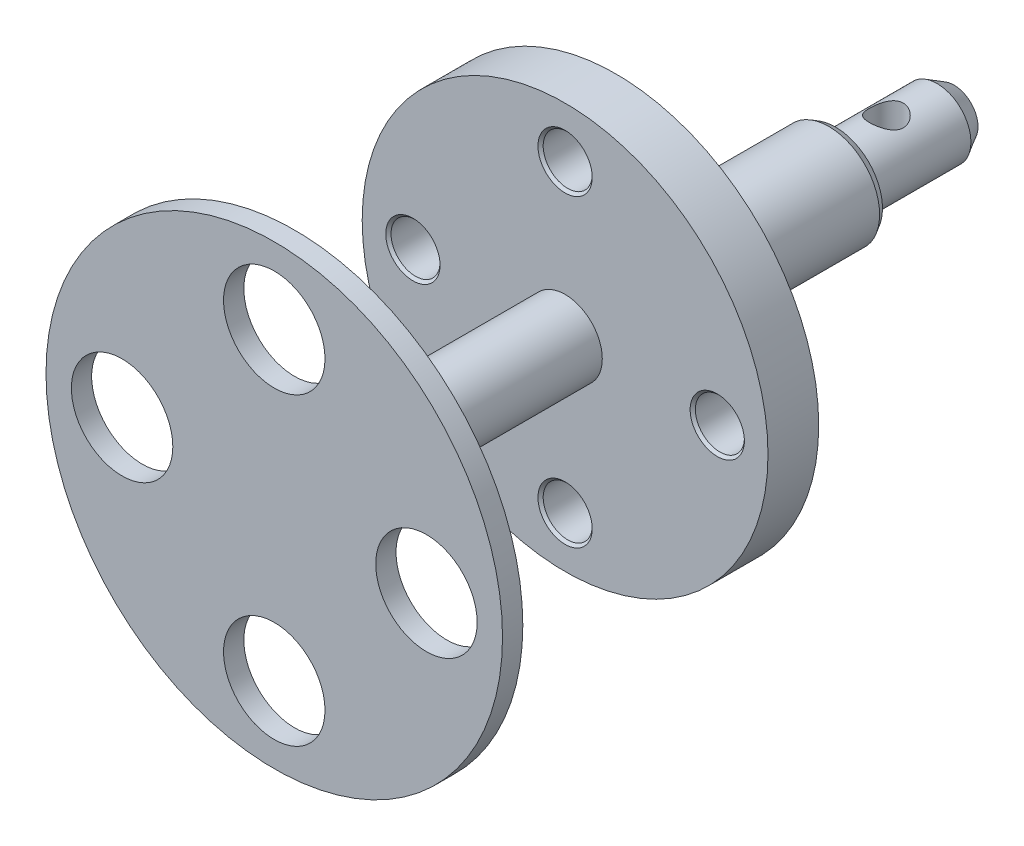
SolidWorks part; units mm, degrees
ref_plane "Front Plane" through (0, 0, 0) normal (0, 0, 1) x (1, 0, 0)
ref_plane "Top Plane" through (0, 0, 0) normal (0, 1, 0) x (1, 0, 0)
ref_plane "Right Plane" through (0, 0, 0) normal (1, 0, 0) x (0, 0, -1)
other "Configuration Table"
sketch "Sketch1" plane through (0, 0, 0) normal (0, 0, 1) x (1, 0, 0)
  circle A0 centre (0, 0) radius 52.5
  circle A1 centre (0, 0) radius 45 construction
  circle A2 centre (0, 45) radius 3.5
  circle A3 centre (38.9711, 22.5) radius 3.5
  circle A4 centre (38.9711, -22.5) radius 3.5
  circle A5 centre (0, -45) radius 3.5
  circle A6 centre (-38.9711, -22.5) radius 3.5
  circle A7 centre (-38.9711, 22.5) radius 3.5
  point P19 (0, 0)
  dimension "D1" = 105
  dimension "D2" = 90
  dimension "D3" = 7
  dimension "D4" = 6
extrude "Boss-Extrude1" add sketch "Sketch1" along normal blind 14
sketch "Sketch2" plane through (0, 0, 14) normal (0, 0, 1) x (1, 0, 0)
  circle A1 centre (0, 0) radius 10
  dimension "D2" = 20
extrude "Boss-Extrude2" add sketch "Sketch2" along normal blind 100
sketch "Sketch3" plane through (0, 0, 114) normal (0, 0, 1) x (1, 0, 0)
  circle A0 centre (0, 0) radius 60
  dimension "D1" = 120
extrude "Boss-Extrude3" add sketch "Sketch3" along normal blind 15
sketch "Sketch4" plane through (0, 0, 129) normal (0, 0, 1) x (1, 0, 0)
  line L0 (0, 0) -> (0, 45) construction
  line L1 (0, 0) -> (-22.5, 38.9711) construction
  circle A0 centre (0, 0) radius 45 construction
  dimension "D1" = 90
  dimension "D2" = 30
hole_wizard "M16x1.5 Tapped Hole1" positions "3DSketch1" profile "Sketch5" tap size "M16x1.5" standard "GB"
sketch3d "3DSketch1"
  point P0 (0, 45, 129)
sketch "Sketch5" plane through (0, 45, 129) normal (1, 0, 0) x (0, -1, 0)
  line L0 (0, 0) -> (0, 40.8562)
  line L1 (0, 40.8562) -> (7.25, 36.5)
  line L2 (7.25, 36.5) -> (7.25, 0.775)
  line L3 (7.25, 0.775) -> (8.025, 0)
  line L5 (8.025, 0) -> (0, 0)
  line L6 (-7.25, 0.775) -> (-8.025, 0) construction
  line L10 (0, 40.8562) -> (-7.25, 36.5) construction
  line L11 (0, -6.35) -> (0, 107.95) construction
  dimension "螺纹孔钻头直径" = 14.5
  dimension "螺纹孔钻头深度" = 36.5
  dimension "近端锥形沉头孔直径" = 16.05
  dimension "近端锥形沉头孔角度" = 90
  dimension "导头角度" = 118
cosmetic thread "Hole Thread 1" parameters "D1"=32, "D2"=16
pattern_circular "CirPattern1" count 4 every 90 about axis through (0, 0, 0) along (0, 0, 1) of "M16x1.5 Tapped Hole1"
sketch "Sketch6" plane through (0, 0, 0) normal (0, 0, -1) x (-1, 0, 0)
  circle A0 centre (0, 0) radius 67.6989
extrude "Cut-Extrude1" cut sketch "Sketch6" against normal blind 14
chamfer "Chamfer1" distance 5 angle 30 1 edges at (-10, 0, 14)
sketch "Sketch7" plane through (0, 0, 0) normal (0, 1, 0) x (1, 0, 0)
  line L0 (7.1132, -14) -> (-7.1132, -14) construction
  circle A0 centre (0, -34) radius 5
  dimension "D1" = 10
  dimension "D2" = 20
extrude "Cut-Extrude2" cut sketch "Sketch7" against normal through all both and the other way through all
sketch "Sketch8" plane through (0, 0, 114) normal (0, 0, -1) x (-1, 0, 0)
  circle A0 centre (0, 0) radius 15
  dimension "D1" = 30
extrude "Boss-Extrude4" add sketch "Sketch8" along normal blind 65
chamfer "Chamfer2" distance 2 angle 30 1 edges at (-15, 0, 49)
sketch "Sketch9" plane through (0, 0, 129) normal (0, 0, 1) x (1, 0, 0)
  circle A0 centre (0, 0) radius 11
  dimension "D1" = 22
extrude "Boss-Extrude5" add sketch "Sketch9" along normal blind 80
sketch "Sketch10" plane through (0, 0, 209) normal (0, 0, 1) x (1, 0, 0)
  circle A0 centre (0, 0) radius 67.5
  circle A1 centre (0, 45) radius 15
  circle A2 centre (45, 0) radius 15
  circle A3 centre (0, -45) radius 15
  circle A4 centre (-45, 0) radius 15
  dimension "D1" = 135
  dimension "D2" = 30
  dimension "D3" = 30
  dimension "D4" = 30
  dimension "D5" = 30
extrude "Boss-Extrude6" add sketch "Sketch10" along normal blind 6
